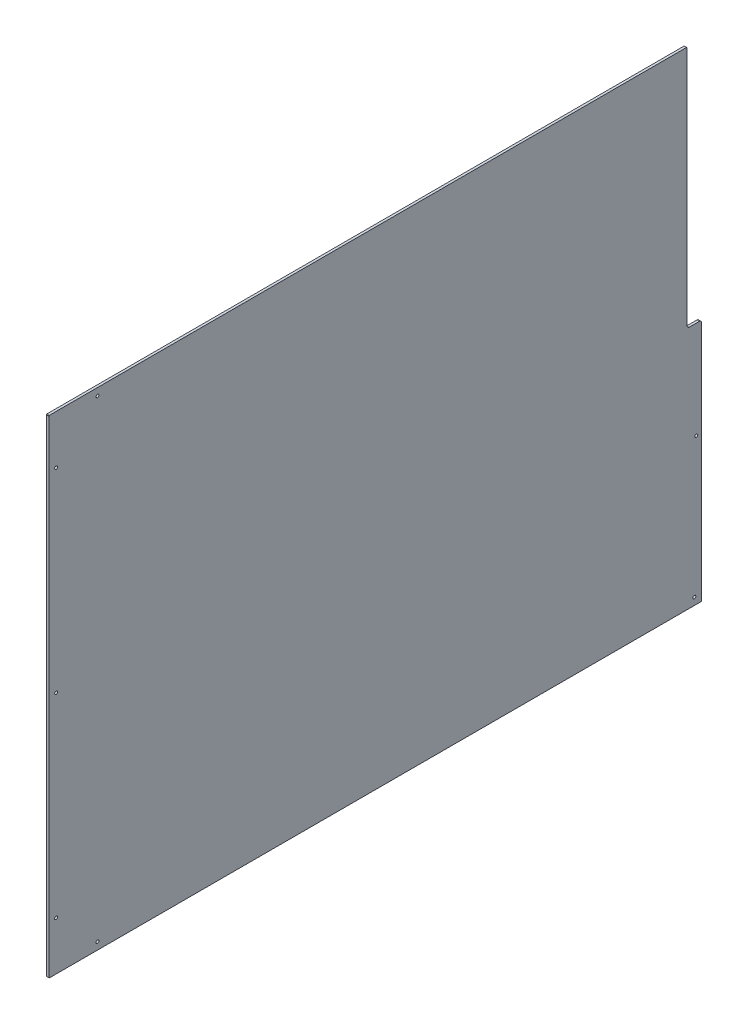
SolidWorks part; units mm, degrees
material "PC(透明)"
ref_plane "前基準面" through (0, 0, 0) normal (0, 0, 1) x (1, 0, 0)
ref_plane "上基準面" through (0, 0, 0) normal (0, 1, 0) x (1, 0, 0)
ref_plane "右基準面" through (0, 0, 0) normal (1, 0, 0) x (0, 0, -1)
sketch "草图1" plane through (0, 0, 0) normal (1, 0, 0) x (0, 0, -1)
  line L1 (670, 500) -> (-670, 500)
  line L2 (670, 500) -> (670, -500)
  line L3 (670, -500) -> (-670, -500)
  line L4 (-670, 500) -> (-670, -500)
  line L5 (670, 500) -> (-670, -500) construction
  line L6 (670, -500) -> (-670, 500) construction
  point P0 (0, 0)
  dimension "D1" = 1340
  dimension "D2" = 1000
extrude "凸台-拉伸1" add sketch "草图1" along normal blind 5
chamfer "倒角1" distance 1 angle 45 4 edges at (2.5, -500, -670) (2.5, -500, 670) (2.5, 500, -670) (2.5, 500, 670)
sketch "草图2" plane through (0, 0, 0) normal (-1, 0, 0) x (0, 0, 1)
  line L0 (-659, 200) -> (-659, -200) construction
  line L1 (-669, 500) -> (669, 500) construction
  line L2 (58.8862, 0) -> (0, 0) construction
  line L3 (0, 0) -> (0, 69.8386) construction
  line L4 (670, 499) -> (670, -499) construction
  line L5 (655, -485) -> (-655, -485) construction
  line L6 (655, -485) -> (655, 485) construction
  line L7 (655, 485) -> (-655, 485) construction
  line L8 (-655, -485) -> (-655, 485) construction
  line L9 (655, -485) -> (-655, 485) construction
  line L10 (655, 485) -> (-655, -485) construction
  line L11 (-669, 500) -> (669, 500) construction
  line L12 (669, -500) -> (-669, -500) construction
  line L13 (-670, -499) -> (-670, 499) construction
  line L14 (-659, 0) -> (-670, 0) construction
  circle A0 centre (-655, 485) radius 3
  circle A1 centre (-655, -485) radius 3
  circle A2 centre (655, -485) radius 3 construction
  circle A3 centre (655, 485) radius 3 construction
  circle A4 centre (570, 485) radius 3
  circle A5 centre (655, 400) radius 3
  circle A6 centre (655, -400) radius 3
  circle A7 centre (570, -485) radius 3
  circle A8 centre (655, 0) radius 3
  circle A9 centre (-655, 0) radius 3 construction
  circle A10 centre (-659, 200) radius 3
  circle A11 centre (-659, -200) radius 3
  dimension "D1" = 6
  dimension "D4" = 100
  dimension "D5" = 100
  dimension "D2" = 15
  dimension "D3" = 15
  dimension "D6" = 100
  dimension "D7" = 15
  dimension "D8" = 11
  dimension "D9" = 400
extrude "切除-拉伸1" cut sketch "草图2" against normal through all
sketch "草图3" plane through (5, 0, 0) normal (1, 0, 0) x (0, 0, -1)
  line L5 (670, 500) -> (640, 500)
  line L6 (670, 500) -> (670, 0)
  line L7 (670, 0) -> (640, 0)
  line L8 (640, 500) -> (640, 0)
  line L10 (669, 500) -> (-669, 500) construction
  line L11 (-669, -500) -> (669, -500) construction
  line L12 (670, -499) -> (670, 499) construction
  dimension "D1" = 30
  dimension "D2" = 500
extrude "切除-拉伸2" cut sketch "草图3" against normal blind 10
chamfer "倒角2" distance 1 angle 45 1 edges at (2.5, 500, -640)
fillet "圆角1" radius 5 1 edges at (2.5, 0, -640)
fillet "圆角2" radius 5 1 edges at (2.5, 0, -670)
